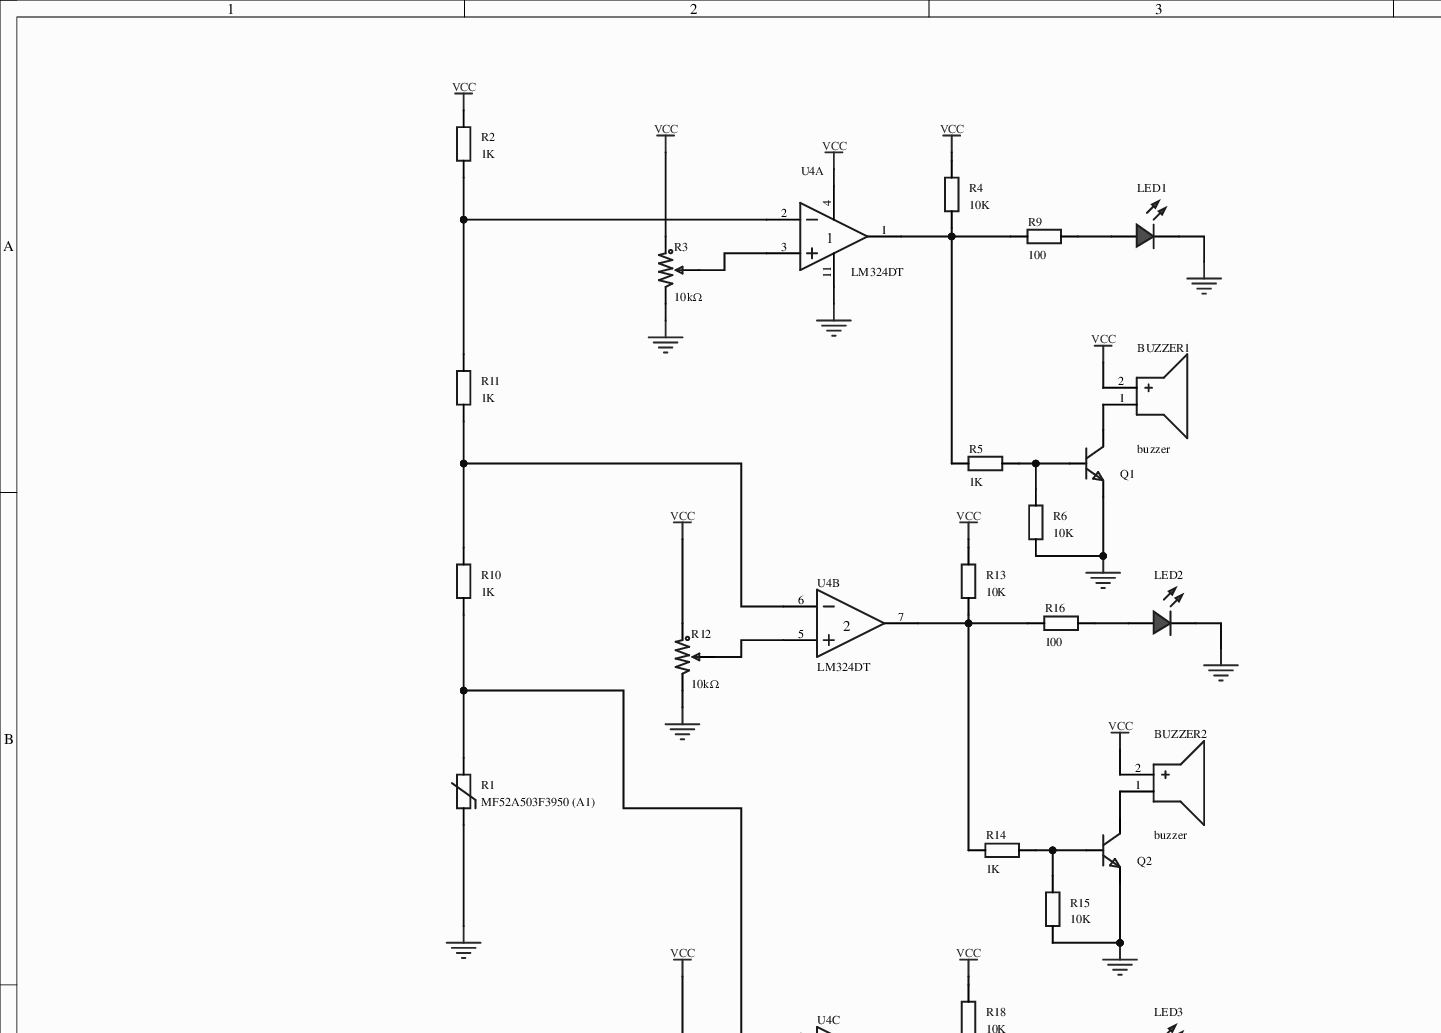
[diagram p0: MISC51921-3.schdoc, top left]
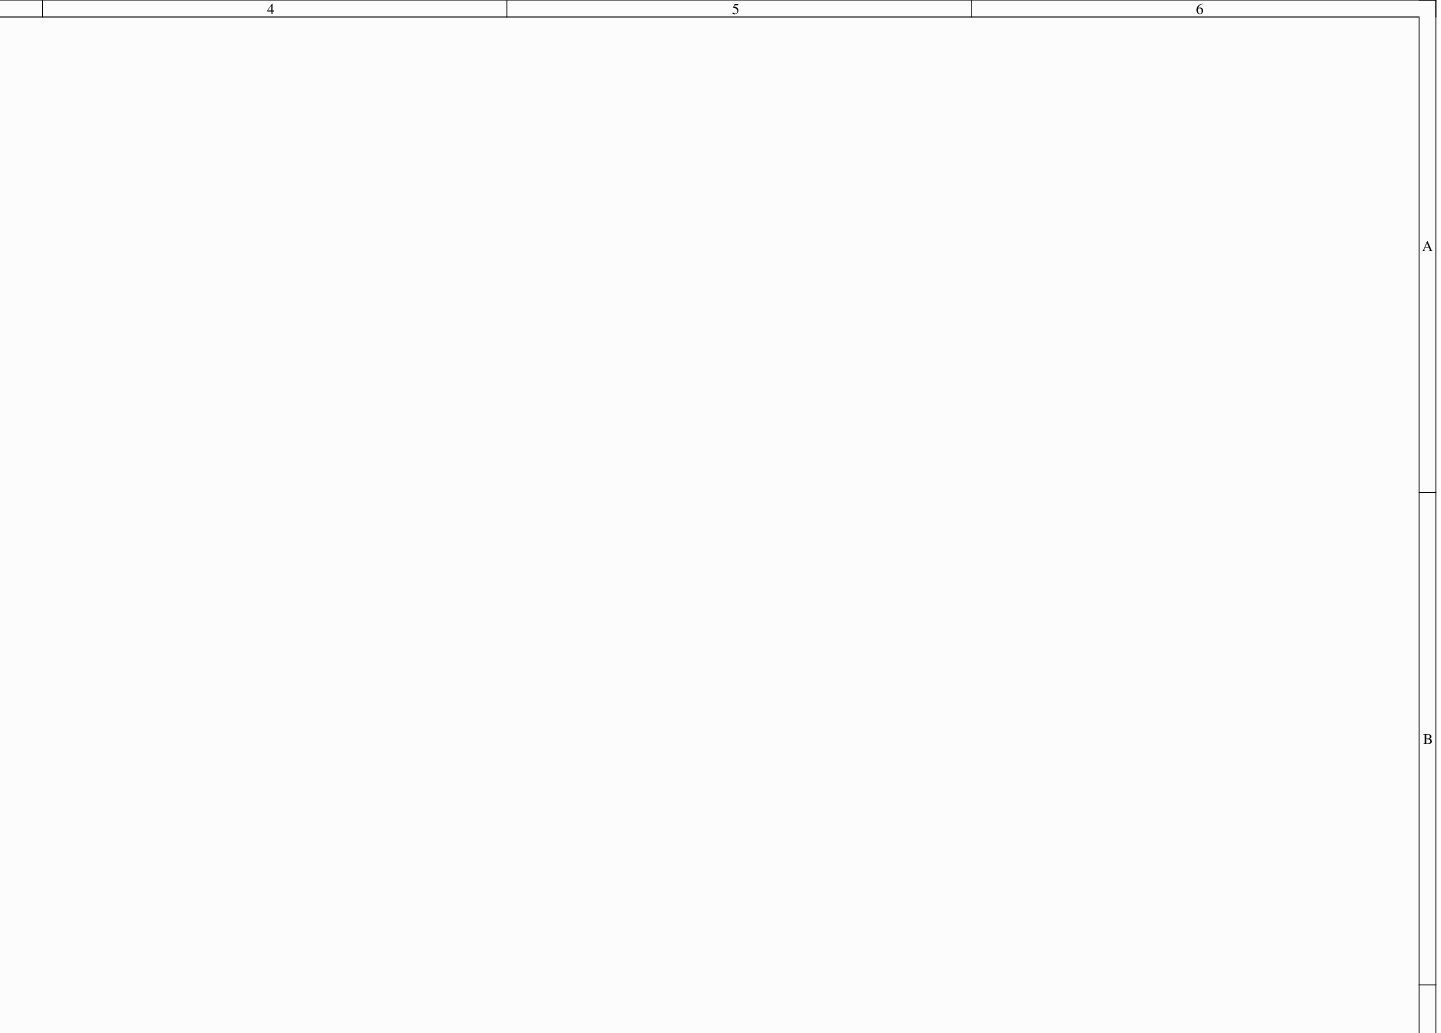
[diagram p1: MISC51921-3.schdoc, top right]
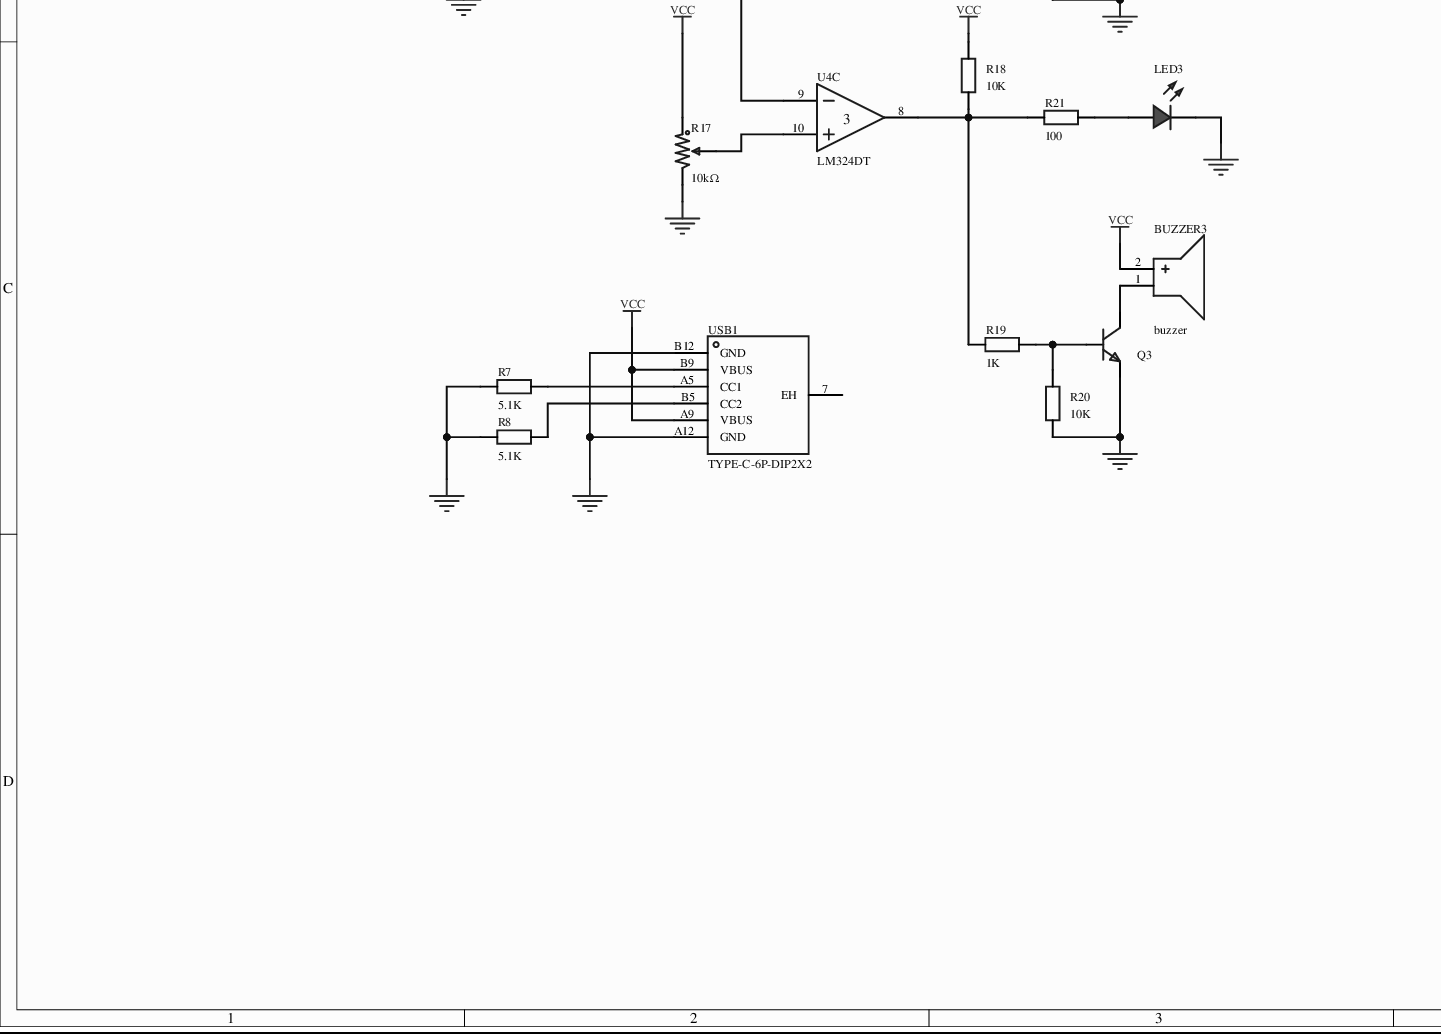
[diagram p2: MISC51921-3.schdoc, bottom left]
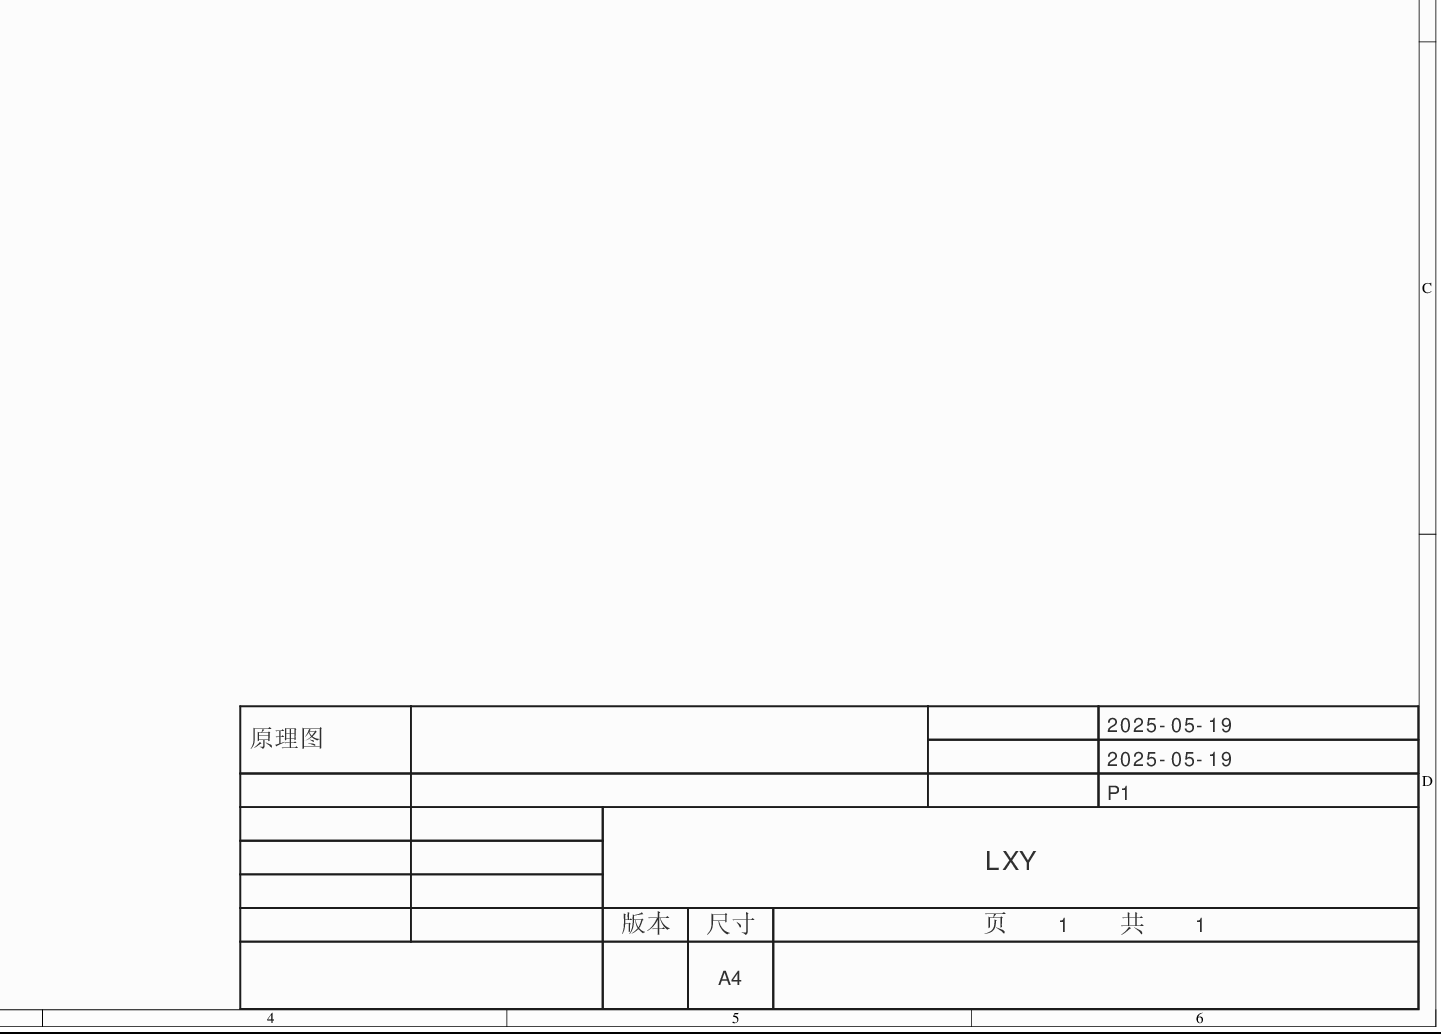
[diagram p3: MISC51921-3.schdoc, bottom right]
# Altium project MISC51921-2.PrjPcb
1 sheet, 32 parts. Net scope: global (net labels, ports and power ports of the same name join across sheets).
Board file: MISC51921.pcbdoc

## Sheet MISC51921-3.schdoc
size 420 x 297 mm; Version: V1.0; @Project Name: MISC51921; @Page Count: 1; @Update Date: 2025-05-19; @Create Date: 2025-05-19; @Schematic Name: MISC51921; @Page No: 1; @Create Time: 14:21:27; @Update Time: 21:36:43; @Board Name: MISC51921

### Parts
BUZZER1  buzzer  [BUZ-TH_BD12.0-P6.00-D0.9-RD]
BUZZER2  buzzer  [BUZ-TH_BD12.0-P6.00-D0.9-RD]
BUZZER3  buzzer  [BUZ-TH_BD12.0-P6.00-D0.9-RD]
LED1  (no value)  [LED_TH-3mm]
LED2  (no value)  [LED_TH-3mm]
LED3  (no value)  [LED_TH-3mm]
Q1  (no value)  [S8050_SOT-23]
Q2  (no value)  [S8050_SOT-23]
Q3  (no value)  [S8050_SOT-23]
R1  MF52A503F3950 (A1)  [RES-TH_L2.5-W2.5-P1.70-D0.3]
R2  1K  [R0603]
R3  10kΩ  [RES-ADJ-SMD_RM065-V1]
R4  10K  [R0603]
R5  1K  [R0603]
R6  10K  [R0603]
R7  5.1K  [R0603]
R8  5.1K  [R0603]
R9  100  [R0603]
R10  1K  [R0603]
R11  1K  [R0603]
R12  10kΩ  [RES-ADJ-SMD_RM065-V1]
R13  10K  [R0603]
R14  1K  [R0603]
R15  10K  [R0603]
R16  100  [R0603]
R17  10kΩ  [RES-ADJ-SMD_RM065-V1]
R18  10K  [R0603]
R19  1K  [R0603]
R20  10K  [R0603]
R21  100  [R0603]
U4  LM324DT  [SOIC-14_L8.7-W3.9-P1.27-LS6.0-BL]  (parts A,B,C of 4)
USB1  TYPE-C-6P-DIP2X2  [TYPE-C-SMD_TYPE-C-6P]

### Nets
GND: LED1.2(A) LED2.2(A) LED3.2(A) Q1.2 Q2.2 Q3.2 R1.1 R3.3 R6.2 R7.1 R8.1 R12.3 R15.2 R17.3 R20.2 U4.11(VCC-) USB1.A12(GND) USB1.B12(GND)
VCC: BUZZER1.2(+) BUZZER2.2(+) BUZZER3.2(+) R2.2 R3.1 R4.2 R12.1 R13.2 R17.1 R18.2 U4.4(VCC+) USB1.A9(VBUS) USB1.B9(VBUS)
NetBUZZER1_1: BUZZER1.1(-) Q1.3
NetBUZZER2_1: BUZZER2.1(-) Q2.3
NetBUZZER3_1: BUZZER3.1(-) Q3.3
NetLED1_1: LED1.1(C) R9.1
NetLED2_1: LED2.1(C) R16.1
NetLED3_1: LED3.1(C) R21.1
NetQ1_1: Q1.1 R5.1 R6.1
NetQ2_1: Q2.1 R14.1 R15.1
NetQ3_1: Q3.1 R19.1 R20.1
NetR1_2: R1.2 R10.1 U4.9(IN3-)
NetR2_1: R2.1 R11.2 U4.2(IN1-)
NetR3_2: R3.2 U4.3(IN1+)
NetR4_1: R4.1 R5.2 R9.2 U4.1(OUT1)
NetR7_2: R7.2 USB1.A5(CC1)
NetR8_2: R8.2 USB1.B5(CC2)
NetR10_2: R10.2 R11.1 U4.6(IN2-)
NetR12_2: R12.2 U4.5(IN2+)
NetR13_1: R13.1 R14.2 R16.2 U4.7(OUT2)
NetR17_2: R17.2 U4.10(IN3+)
NetR18_1: R18.1 R19.2 R21.2 U4.8(OUT3)

Not connected (* = marked no-connect by the designer): USB1 7(EH)

### Notes on the sheet
- 2025-05-19
- 原理图
- P1
- LXY
- 版本
- 尺寸
- A4
- 页    1    共    1

### Library data of the parts
BUZZER1-BUZZER3 = buzzer: AddInBom: yes; ModelId: af17e4151ed84fc2a628230bf2376363; ModelTransform: 472.44,472.176,0,270,0,0,0,0,-196.85; Symbol: BUZZER; Device: buzzer; LCSC Part Name: buzzer; SupplierPart: C9900014030; ManufacturerPart: buzzer; Supplier Footprint: buzzer; Supplier: LCSC; ConvertToPcb: yes; FootprintName: BUZ-TH_BD12.0-P6.00-D0.9-RD; ModelName: BUZ-TH_BD12.0-P6.00-D0.9-RD
LED1-LED3 = LED_TH-R_3mm: ConvertToPcb: yes; ModelId: a497c992633541038a38947cdc58012f; ModelName: LED-TH-3mm_R; ModelTransform: 141.274,153.327,0,0,0,0,-5.984,0,-137.795; Symbol: LED_TH-R; Device: LED_TH-R_3mm; AddInBom: yes; FootprintName: LED_TH-3mm; Supplier Footprint: 插件
Q1-Q3 = S8050_SOT_NPN: ConvertToPcb: yes; SymbolName: NPN; ModelId: c62791f0466c4ae2a892c056b845b0ca; ModelName: SOT-23-3P_L2.9-W1.3-H1.0-LS2.4-P0.95; ModelTransform: 98.6,114.12,41.29,180,0,0,0,0,-3; Device: S8050_SOT_NPN; AddInBom: yes; Supplier Footprint: SOT-23; FootprintName: S8050_SOT-23
R1 = MF52A503F3950 (A1): 阻值:50kΩ;B值(25℃/50℃):3950K;功率:50mW;B值精度:±1%;最大稳态电流(25℃):-;; Manufacturer: 时恒; Symbol: 50KΩ ±1%; AddInBom: yes; ModelId: ca46172ea1764ea88d6c38442d1f6f09; ModelName: RES-TH_L2.5-W2.5-P1.70; ModelTransform: 98.425,98.2987,0,0,0,0,0,0,-118.11; Resistance @ 25℃: 50kΩ; B Constant (25℃/50℃): 3950K; Power(Watts): 50mW; B Constant Tolerance: ±1%; Device: MF52A503F3950 (A1); LCSC Part Name: MF52A503F3950 (A1); SupplierPart: C123379; ManufacturerPart: MF52A503F3950 (A1); Supplier Footprint: 插件,P=1.7mm; Datasheet: https://atta.szlcsc.com/upload/public/pdf/source/20170728/C123379_1501225823221848942.pdf; Supplier: LCSC; ConvertToPcb: yes; FootprintName: RES-TH_L2.5-W2.5-P1.70-D0.3; B Constant (25℃/75℃): -; B Constant (25℃/85℃): -; B Constant (25℃/100℃): -; Steady State Current (Max): -; Operating Temperature: -55℃~+125℃
R2 R4-R11 R13-R16 R18-R21 = Res_0603: ConvertToPcb: yes; SymbolName: 电阻; ModelId: fc143cca1e79419f9cd78b61e9279f08; ModelTransform: 31.8897,63.7794,0,90,0,0,0,0,0; Device: Res_0603; AddInBom: yes; Supplier Footprint: 0603; FootprintName: R0603; ModelName: R0603
  R2 R5 R10 R11 R14 R19: Value: 1K
  R4 R6 R13 R15 R18 R20: Value: 10K
  R7 R8: Value: 5.1K
  R9 R16 R21: Value: 100
R3 R12 R17 = RM065-103(10K): 阻值:10kΩ;精度:±25%;功率:100mW;; Manufacturer: BOCHEN(博晨); AddInBom: yes; ModelId: c816c2b7942147f5a832150e8ef6960c; ModelTransform: 255.905,283.464,0,0,0,0,0.025,-3.937,-157.48; Tolerance: ±25%; Power(Watts): 100mW; Symbol: RM065-103(10K); Device: RM065-103(10K); LCSC Part Name: 10kΩ ±25%; SupplierPart: C5205021; ManufacturerPart: RM065-103(10K); Supplier Footprint: 插件; JLCPCB Part Class: Extended Part; Datasheet: https://atta.szlcsc.com/upload/public/pdf/source/20221019/6263C46FBC7F1B66CBAADA74DC5EFAA2.pdf; Supplier: LCSC; ConvertToPcb: yes; FootprintName: RES-ADJ-SMD_RM065-V1; ModelName: RES-ADJ-SMD_RM065-V1; Value: 10kΩ
U4 = LM324DT: 放大器数:四路;轨到轨:-;增益带宽积(GBP):-;输入失调电压(Vos):5mV;压摆率(SR):20V/us;输入偏置电流(Ib):300nA;; Manufacturer: ST(意法半导体); Relevance: []; AddInBom: yes; ModelId: 8dbf5b715d42428c85558507ae5a252b; ModelName: SOIC-14_L8.6-W3.9-H1.8-LS6.0-P1.27; ModelTransform: 338.583,236.22,0,0,0,0,0,-0.001,0; Number of Channels: 四路; Maximum Power Supply Range (Vdd-Vss): 30V; Vos - Input Offset Voltage: 5mV; Input Offset Voltage Drift(Vos TC): 30uV/℃; Slew Rate: 20V/us; Ib - Input Bias Current: 300nA; Noise density(eN): 40nV/√Hz@1kHz; Common Mode Rejection Ratio(CMRR): 80dB; Single supply: 3V~30V; Dual Supply: -15V~-1.5V；1.5V~15V; Symbol: LM324DT; Device: LM324DT; LCSC Part Name: LM324DT; SupplierPart: C71035; ManufacturerPart: LM324DT; Supplier Footprint: SOIC-14; Datasheet: https://atta.szlcsc.com/upload/public/pdf/source/20191009/C435836_73A2A70B7EBF6488ECBA427A13AA28C8.pdf; Supplier: LCSC; ConvertToPcb: yes; FootprintName: SOIC-14_L8.7-W3.9-P1.27-LS6.0-BL; Rail to Rail: -; Gain Bandwidth Product: -; Input Offset Current(Ios): -; Input offset current drift(Ios TC): -; Quiescent Current: -; Output Current: -; Operating Temperature: 0℃~+70℃
USB1 = TYPE-C-6P-DIP2X2: AddInBom: yes; ModelId: 3770c5585474407db939b2377e27177a; ModelName: TYPE-C-SMD_6P-L8.9-W6.8-H3.2-P1.00; ModelTransform: 351.9678,267.716,0,180,0,0,0,-48.226,-39.37; Symbol: TYPE-C-6P-DIP2X2; Device: TYPE-C-6P-DIP2X2; LCSC Part Name: TYPE-C-6P-DIP2X2; SupplierPart: C9900017627; ManufacturerPart: TYPE-C-6P-DIP2X2; Supplier Footprint: TYPE-C-6P; JLCPCB Part Class: 扩展库; Supplier: LCSC; ConvertToPcb: yes; FootprintName: TYPE-C-SMD_TYPE-C-6P